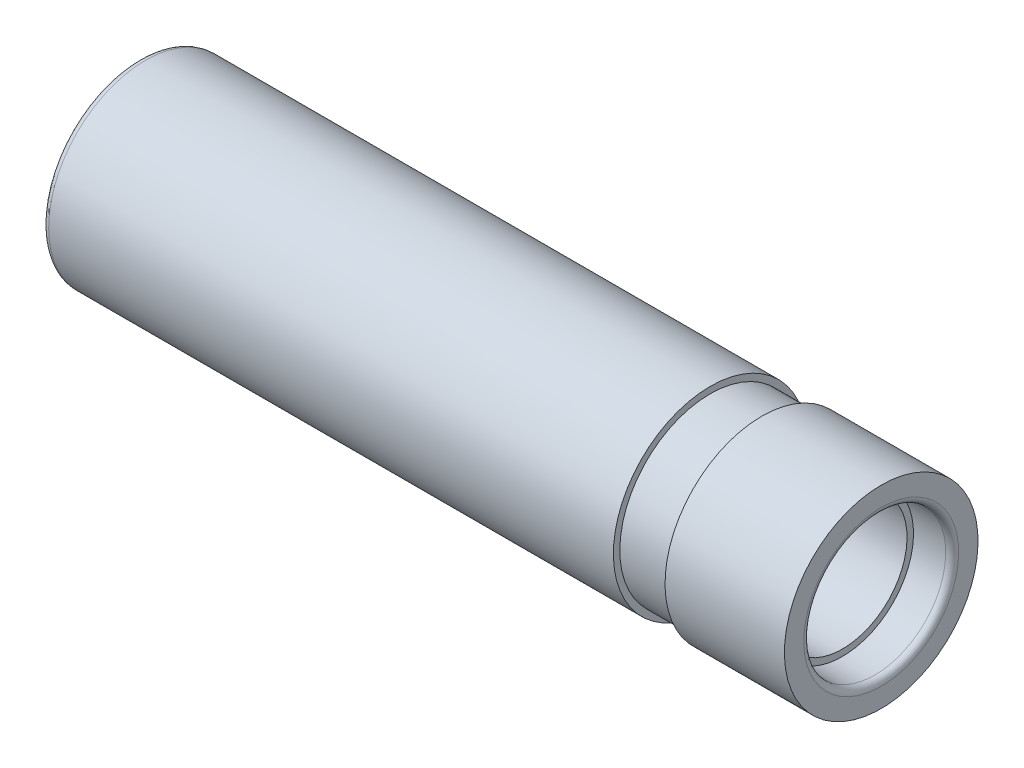
SolidWorks part; units mm, degrees
ref_plane "Front Plane" through (0, 0, 0) normal (0, 0, 1) x (1, 0, 0)
ref_plane "Top Plane" through (0, 0, 0) normal (0, 1, 0) x (1, 0, 0)
ref_plane "Right Plane" through (0, 0, 0) normal (1, 0, 0) x (0, 0, -1)
sketch "Sketch1" plane through (0, 0, 0) normal (0, 0, 1) x (1, 0, 0)
  line L0 (-54.5696, 7.7573) -> (-54.5696, 11.7702)
  line L1 (-54.5696, 11.7702) -> (33.9304, 11.7702)
  line L2 (60.4304, 11.7702) -> (60.4304, 7.7702)
  line L3 (54.4304, -3.2298) -> (-48.5696, -3.2298) construction
  line L4 (-54.5696, 7.7573) -> (-48.5696, 7.7573)
  line L5 (-48.5696, 7.7573) -> (-48.5696, 6.7702)
  line L6 (60.4304, 7.7702) -> (54.4304, 7.7702)
  line L7 (54.4304, 7.7702) -> (54.4304, 6.7702)
  line L8 (-48.5696, 6.7702) -> (54.4304, 6.7702)
  line L9 (41.9304, 11.7702) -> (41.9304, 10.7702)
  line L10 (41.9304, 10.7702) -> (33.9304, 10.7702)
  line L11 (33.9304, 10.7702) -> (33.9304, 11.7702)
  line L12 (41.9304, 11.7702) -> (60.4304, 11.7702)
  dimension "D1" = 115
  dimension "D2" = 15
  dimension "D3" = 11
  dimension "D4" = 10
  dimension "D5" = 6
  dimension "D6" = 6
  dimension "D7" = 18.5
  dimension "D8" = 8
  dimension "D9" = 1
revolve "Revolve1" add sketch "Sketch1" angle 360 about L3
fillet "Fillet1" radius 1 3 edges at (60.4304, 7.7702, 0) (-54.5696, 11.7702, 0) (-54.5696, 7.7573, 0)
